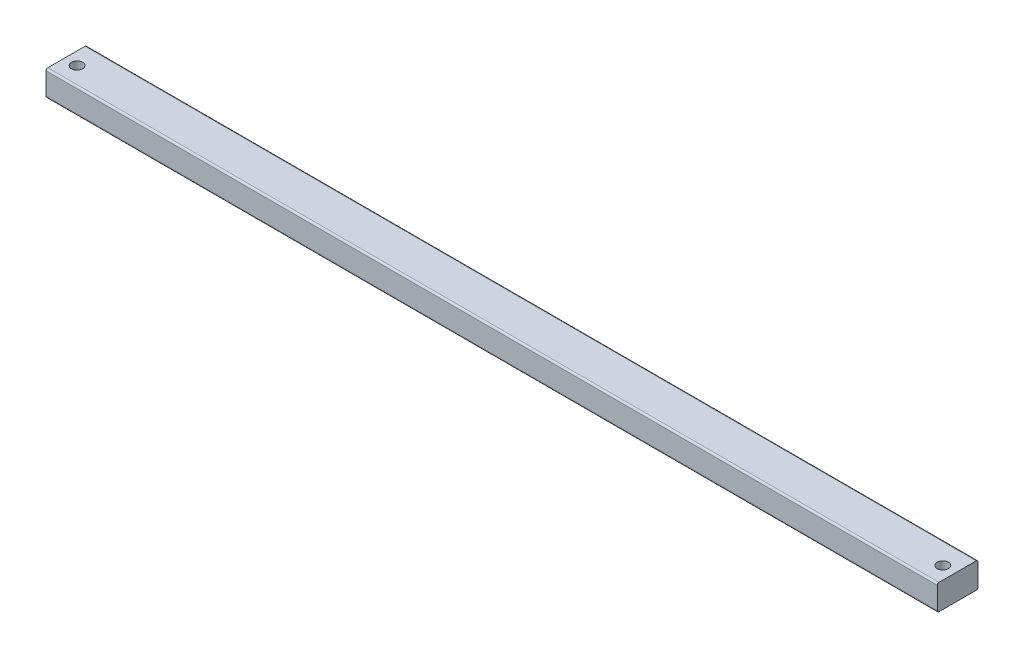
SolidWorks part; units mm, degrees
ref_plane "Front Plane" through (0, 0, 0) normal (0, 0, 1) x (1, 0, 0)
ref_plane "Top Plane" through (0, 0, 0) normal (0, 1, 0) x (1, 0, 0)
ref_plane "Right Plane" through (0, 0, 0) normal (1, 0, 0) x (0, 0, -1)
sketch "Sketch1" plane through (0, 0, 0) normal (0, 0, 1) x (1, 0, 0)
  line L0 (-32.1938, 0) -> (842.8062, 0)
  dimension "D1" = 875
ref_plane "Plane1" through (-32.1938, 0, 0) normal (1, 0, 0) x (0, 0, -1)
sketch "Sketch2" plane through (-32.1938, 0, 0) normal (1, 0, 0) x (0, 0, -1)
  line L1 (20, 12.5) -> (-20, 12.5)
  line L2 (20, 12.5) -> (20, -12.5)
  line L3 (20, -12.5) -> (-20, -12.5)
  line L4 (-20, 12.5) -> (-20, -12.5)
  line L5 (20, 12.5) -> (-20, -12.5) construction
  line L6 (20, -12.5) -> (-20, 12.5) construction
  point P0 (0, 0)
  dimension "D1" = 40
  dimension "D2" = 25
sweep "Sweep1" add profiles "Sketch2" path "Sketch1"
fillet "Fillet1" radius 1.7 4 edges at (405.3062, -12.5, -20) (405.3062, -12.5, 20) (405.3062, 12.5, 20) (405.3062, 12.5, -20)
sketch "Sketch3" plane through (0, -12.5, 0) normal (0, -1, 0) x (-1, 0, 0)
  line L0 (32.1938, -18.3) -> (32.1938, 18.3) construction
  line L1 (32.1938, -20) -> (-842.8062, -20) construction
  line L2 (-405.3062, -18.3) -> (-405.3062, 18.3) construction
  line L3 (-842.8062, -18.3) -> (32.1938, -18.3) construction
  line L4 (32.1938, 18.3) -> (-842.8062, 18.3) construction
  circle A0 centre (19.6938, -2) radius 5.5
  circle A1 centre (-830.3062, -2) radius 5.5
  dimension "D1" = 12.5
  dimension "D2" = 18
extrude "Cut-Extrude1" cut sketch "Sketch3" against normal through all
